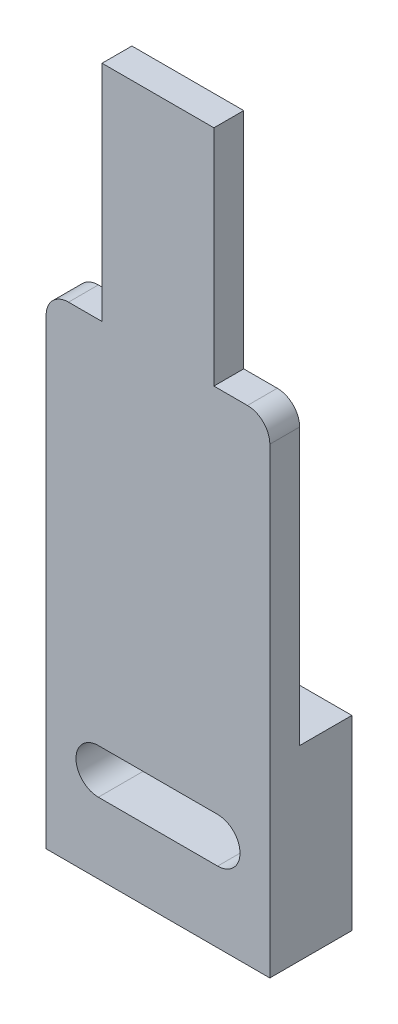
SolidWorks part; units mm, degrees
ref_plane "前视基准面" through (0, 0, 0) normal (0, 0, 1) x (1, 0, 0)
ref_plane "上视基准面" through (0, 0, 0) normal (0, 1, 0) x (1, 0, 0)
ref_plane "右视基准面" through (0, 0, 0) normal (1, 0, 0) x (0, 0, -1)
sketch "草图1" plane through (0, 0, 0) normal (0, 0, 1) x (1, 0, 0)
  line L0 (0, 0) -> (-15, 0)
  line L1 (-15, 0) -> (-15, 25)
  line L2 (-15, 25) -> (15, 25)
  line L7 (15, 25) -> (15, 0)
  line L8 (15, 0) -> (0, 0)
  line L9 (-8, 12.5) -> (8, 12.5) construction
  line L10 (-8, 15.5) -> (8, 15.5)
  line L11 (-8, 9.5) -> (8, 9.5)
  arc A0 (-8, 15.5) -> (-8, 9.5) centre (-8, 12.5) ccw
  arc A1 (8, 9.5) -> (8, 15.5) centre (8, 12.5) ccw
  point P11 (0, 12.5)
  dimension "D5" = 3
  dimension "D1" = 25
  dimension "D2" = 30
  dimension "D6" = 12.5
  dimension "D7" = 16
extrude "凸台-拉伸1" add sketch "草图1" along normal blind 7
sketch "草图2" plane through (0, 0, 7) normal (0, 0, 1) x (1, 0, 0)
  line L0 (-8, 9.5) -> (8, 9.5) construction
  line L1 (-15, 0) -> (15, 0)
  line L2 (-15, 0) -> (-15, 65)
  line L3 (-15, 65) -> (15, 65)
  line L4 (15, 0) -> (15, 65)
  line L5 (8, 15.5) -> (-8, 15.5) construction
  line L6 (-8, 9.5) -> (8, 9.5)
  line L7 (8, 15.5) -> (-8, 15.5)
  arc A0 (8, 9.5) -> (8, 15.5) centre (8, 12.5) ccw construction
  arc A1 (-8, 15.5) -> (-8, 9.5) centre (-8, 12.5) ccw construction
  arc A2 (8, 9.5) -> (8, 15.5) centre (8, 12.5) ccw
  arc A3 (-8, 15.5) -> (-8, 9.5) centre (-8, 12.5) ccw
  dimension "D1" = 65
extrude "凸台-拉伸2" add sketch "草图2" along normal blind 4
fillet "圆角1" radius 3 2 edges at (15, 65, 9) (-15, 65, 9)
sketch "草图3" plane through (0, 0, 11) normal (0, 0, 1) x (1, 0, 0)
  line L0 (-7.5, 65) -> (-7.5, 95)
  line L1 (12, 65) -> (-12, 65) construction
  line L2 (-7.5, 95) -> (7.5, 95)
  line L3 (7.5, 95) -> (7.5, 65)
  line L4 (7.5, 65) -> (-7.5, 65)
  line L5 (0, 65) -> (0, 0) construction
  dimension "D1" = 15
  dimension "D2" = 30
extrude "凸台-拉伸3" add sketch "草图3" against normal up to surface (4 mm away) up to face at (0, 50.8738, 7)
